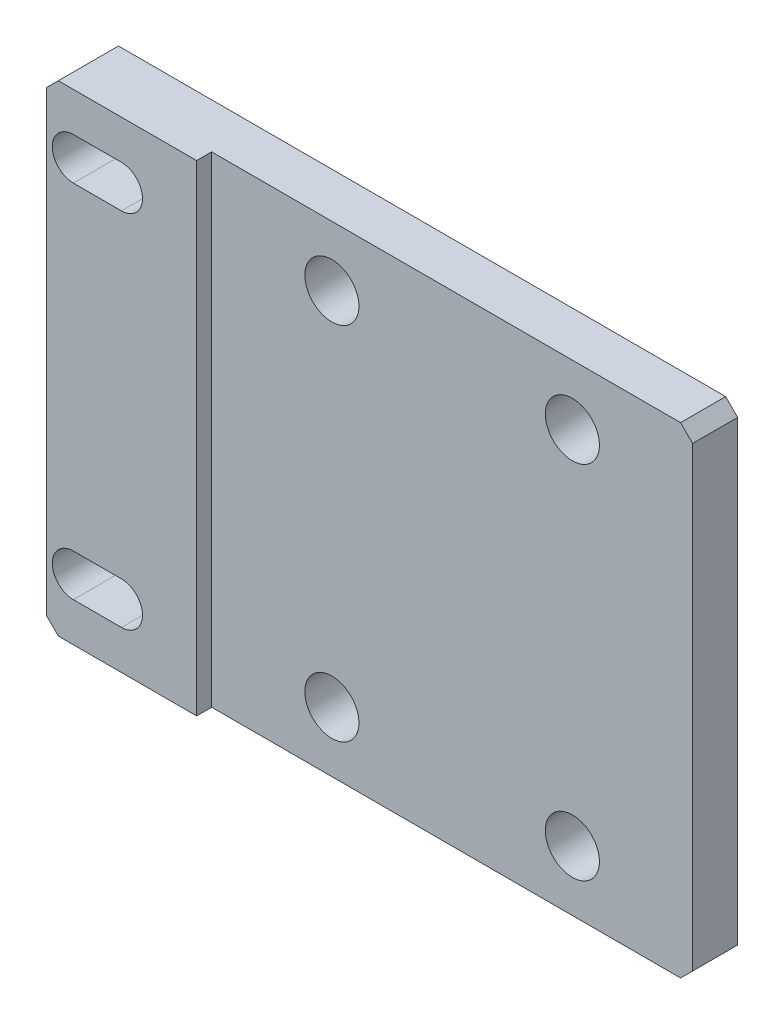
SolidWorks part; units mm, degrees
ref_plane "前视基准面" through (0, 0, 0) normal (0, 0, 1) x (1, 0, 0)
ref_plane "上视基准面" through (0, 0, 0) normal (0, 1, 0) x (1, 0, 0)
ref_plane "右视基准面" through (0, 0, 0) normal (1, 0, 0) x (0, 0, -1)
sketch "草图1" plane through (0, 0, 0) normal (0, 0, 1) x (1, 0, 0)
  line L1 (-52.5, 40) -> (52.5, 40)
  line L2 (-52.5, 40) -> (-52.5, -40)
  line L3 (-52.5, -40) -> (52.5, -40)
  line L4 (52.5, 40) -> (52.5, -40)
  line L5 (-52.5, 40) -> (52.5, -40) construction
  line L6 (-52.5, -40) -> (52.5, 40) construction
  point P0 (0, 0)
  dimension "D1" = 105
  dimension "D2" = 80
extrude "凸台-拉伸1" add sketch "草图1" along normal mid plane 10
sketch "草图2" plane through (0, 0, 5) normal (0, 0, 1) x (1, 0, 0)
  line L0 (-52.5, -40) -> (52.5, -40) construction
  line L1 (52.5, 40) -> (-27.5, 40)
  line L2 (52.5, 40) -> (52.5, -40)
  line L3 (52.5, -40) -> (-27.5, -40)
  line L4 (-27.5, 40) -> (-27.5, -40)
  dimension "D1" = 80
extrude "切除-拉伸1" cut sketch "草图2" against normal blind 2.5
hole_wizard "Ø9.0 (9) 直径孔1" positions "草图4" profile "草图3" hole size "Ø9.0" standard "ISO" end condition through all
sketch "草图4" plane through (0, 0, 5) normal (0, 0, 1) x (1, 0, 0)
  line L0 (52.5, -40) -> (52.5, 40) construction
  line L1 (-3.9923, 0) -> (72.0871, 0) construction
  point P7 (-7.5, 30)
  point P9 (32.5, 30)
  point P20 (32.5, -30)
  point P21 (-7.5, -30)
  dimension "D1" = 20
  dimension "D2" = 40
  dimension "D3" = 30
sketch "草图3" plane through (-7.5, 30, 5) normal (1, 0, 0) x (0, -1, 0)
  line L0 (0, 0) -> (0, 10)
  line L1 (0, 10) -> (4.5, 10)
  line L2 (4.5, 10) -> (4.5, 0)
  line L5 (4.5, 0) -> (0, 0)
  line L11 (0, -6.35) -> (0, 107.95) construction
  dimension "通孔孔直径" = 9
  dimension "通孔孔深度" = 10
hole_wizard "Ø7.0 (7) 直径孔1" positions "草图6" profile "草图5" hole size "Ø7.0" standard "ISO" end condition through all
sketch "草图6" plane through (0, 0, 5) normal (0, 0, 1) x (1, 0, 0)
  line L0 (0, 0) -> (-64.1025, 0) construction
  circle A0 centre (-7.5, 30) radius 4.5 construction
  point P0 (-44, 30)
  point P2 (-86, 30)
  point P13 (-44, -30)
  point P14 (-86, -30)
  dimension "D1" = 36.5
  dimension "D2" = 42
  dimension "D3" = 30
sketch "草图5" plane through (-44, 30, 5) normal (1, 0, 0) x (0, -1, 0)
  line L0 (0, 0) -> (0, 10)
  line L1 (0, 10) -> (3.5, 10)
  line L2 (3.5, 10) -> (3.5, 0)
  line L5 (3.5, 0) -> (0, 0)
  line L11 (0, -6.35) -> (0, 107.95) construction
  dimension "通孔孔直径" = 7
  dimension "通孔孔深度" = 10
chamfer "倒角1" distance 2 angle 45 4 edges at (-52.5, -40, 0) (-52.5, 40, 0) (52.5, 40, -1.25) (52.5, -40, -1.25)
sketch "草图8" plane through (0, 0, 5) normal (0, 0, 1) x (1, 0, 0)
  line L0 (-40, 30) -> (-48, 30) construction
  line L1 (-40, 26.5) -> (-48, 26.5)
  line L2 (-40, 33.5) -> (-48, 33.5)
  arc A0 (-40, 26.5) -> (-40, 33.5) centre (-40, 30) ccw
  arc A1 (-48, 33.5) -> (-48, 26.5) centre (-48, 30) ccw
  circle A2 centre (-44, 30) radius 3.5 construction
  point P2 (-44, 30)
  dimension "D1" = 8
extrude "切除-拉伸3" cut sketch "草图8" against normal blind 10
pattern_linear "阵列(线性)1" count 2 spacing 60 along (0, -1, 0) of "切除-拉伸3"
